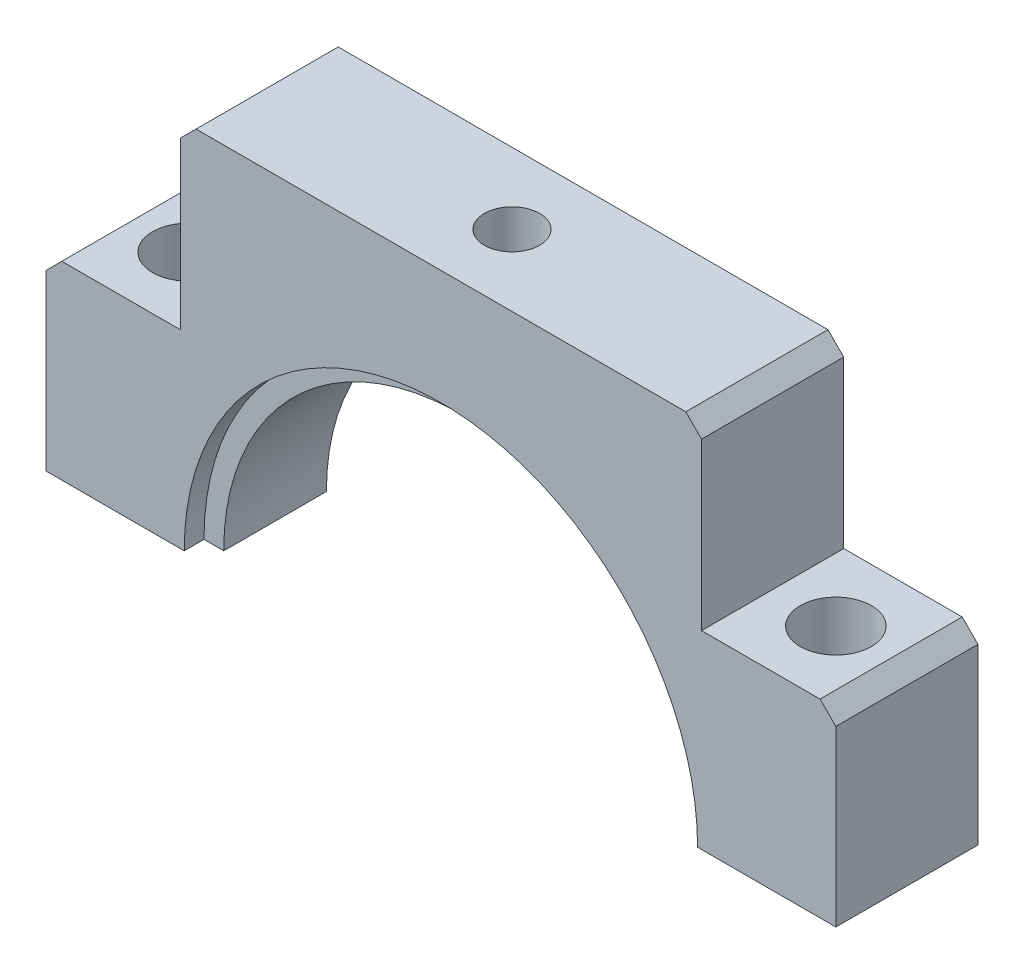
from build123d import *

# Parameters (mm, degrees)
BOSS_EXTRUDE1_DEPTH       = 18
CHAMFER1_SIZE             = 2
M8X1_0_TAPPED_HOLE1_D     = 7
M8X1_0_TAPPED_HOLE1_DEPTH = 13
M8X1_0_TAPPED_HOLE1_TIP   = 2.103012167
HOLE2_D                   = 9
SKETCH15_R                = 32.5
CUT_EXTRUDE3_DEPTH        = 2.5
CUT_EXTRUDE4_START        = -2.5
SKETCH16_R                = 32.5
CUT_EXTRUDE4_DEPTH        = 2.5
HOLE3_D                   = 4


with BuildPart() as part:
    # Sketch1 → Boss-Extrude1 (new body)
    with BuildSketch(Plane.XY):
        with BuildLine():
            Line((-50, 24), (-33, 24))
            Line((-33, 24), (-33, 47))
            Line((-33, 47), (33, 47))
            Line((33, 47), (33, 24))
            Line((33, 24), (50, 24))
            Line((50, 24), (50, 0))
            Line((50, 0), (30, 0))
            ThreePointArc((30, 0), (0, 30), (-30, 0))
            Line((-30, 0), (-50, 0))
            Line((-50, 0), (-50, 24))
        make_face()
    extrude(amount=BOSS_EXTRUDE1_DEPTH)

    # Chamfer1
    chamfer1_edges = [part.edges().sort_by_distance(p)[0] for p in [
        (-50, 24, 9),
        (-33, 47, 9),
        (33, 47, 9),
        (50, 24, 9),
    ]]
    chamfer(chamfer1_edges, length=CHAMFER1_SIZE)

    # M8x1.0 Tapped Hole1
    with Locations(Plane(origin=(0, 47, 0), x_dir=(1, 0, 0), z_dir=(0, 1, 0))):
        with Locations((0, -9)):
            Hole(M8X1_0_TAPPED_HOLE1_D / 2, depth=M8X1_0_TAPPED_HOLE1_DEPTH)
            with Locations((0, 0, -(M8X1_0_TAPPED_HOLE1_DEPTH + M8X1_0_TAPPED_HOLE1_TIP / 2))):  # 118° drill point
                Cone(0, M8X1_0_TAPPED_HOLE1_D / 2, M8X1_0_TAPPED_HOLE1_TIP, mode=Mode.SUBTRACT)

    # Hole2 (through all)
    with Locations(Plane(origin=(0, 24, 0), x_dir=(1, 0, 0), z_dir=(0, 1, 0))):
        with Locations((-41, -9), (41, -9)):
            Hole(HOLE2_D / 2)

    # Sketch15 → Cut-Extrude3 (cut)
    with BuildSketch(Plane(origin=(0, 0, 0), x_dir=(-1, 0, 0), z_dir=(0, 0, -1))):
        Circle(SKETCH15_R)
    extrude(amount=-CUT_EXTRUDE3_DEPTH, mode=Mode.SUBTRACT)

    # Sketch16 → Cut-Extrude4 (cut)
    with BuildSketch(Plane.XY.offset(18).offset(CUT_EXTRUDE4_START)):
        Circle(SKETCH16_R)
    extrude(amount=CUT_EXTRUDE4_DEPTH, mode=Mode.SUBTRACT)

    # Hole3 (through all)
    with Locations(Plane(origin=(0, 47, 0), x_dir=(1, 0, 0), z_dir=(0, 1, 0))):
        with Locations((0, -9)):
            Hole(HOLE3_D / 2)


solid = part.part
